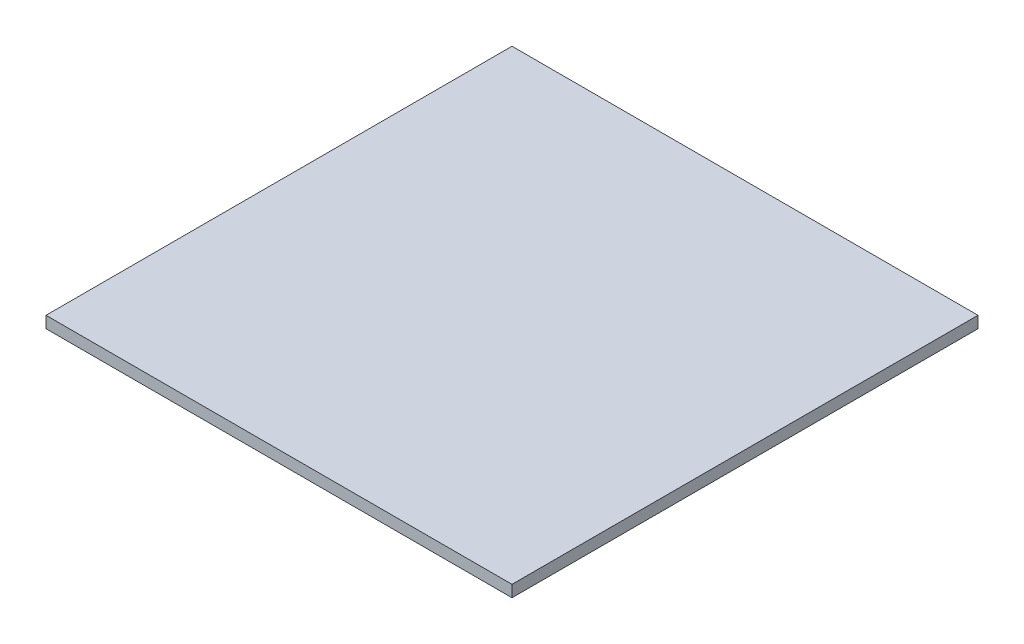
SolidWorks part; units mm, degrees
ref_plane "Front Plane" through (0, 0, 0) normal (0, 0, 1) x (1, 0, 0)
ref_plane "Top Plane" through (0, 0, 0) normal (0, 1, 0) x (1, 0, 0)
ref_plane "Right Plane" through (0, 0, 0) normal (1, 0, 0) x (0, 0, -1)
sketch "Sketch1" plane through (0, 0, 0) normal (0, 1, 0) x (1, 0, 0)
  line L1 (-40, 40) -> (40, 40)
  line L2 (-40, 40) -> (-40, -40)
  line L3 (-40, -40) -> (40, -40)
  line L4 (40, 40) -> (40, -40)
  line L5 (-40, 40) -> (40, -40) construction
  line L6 (-40, -40) -> (40, 40) construction
  point P0 (0, 0)
  dimension "D1" = 80
  dimension "D2" = 80
extrude "Boss-Extrude1" add sketch "Sketch1" along normal blind 2
